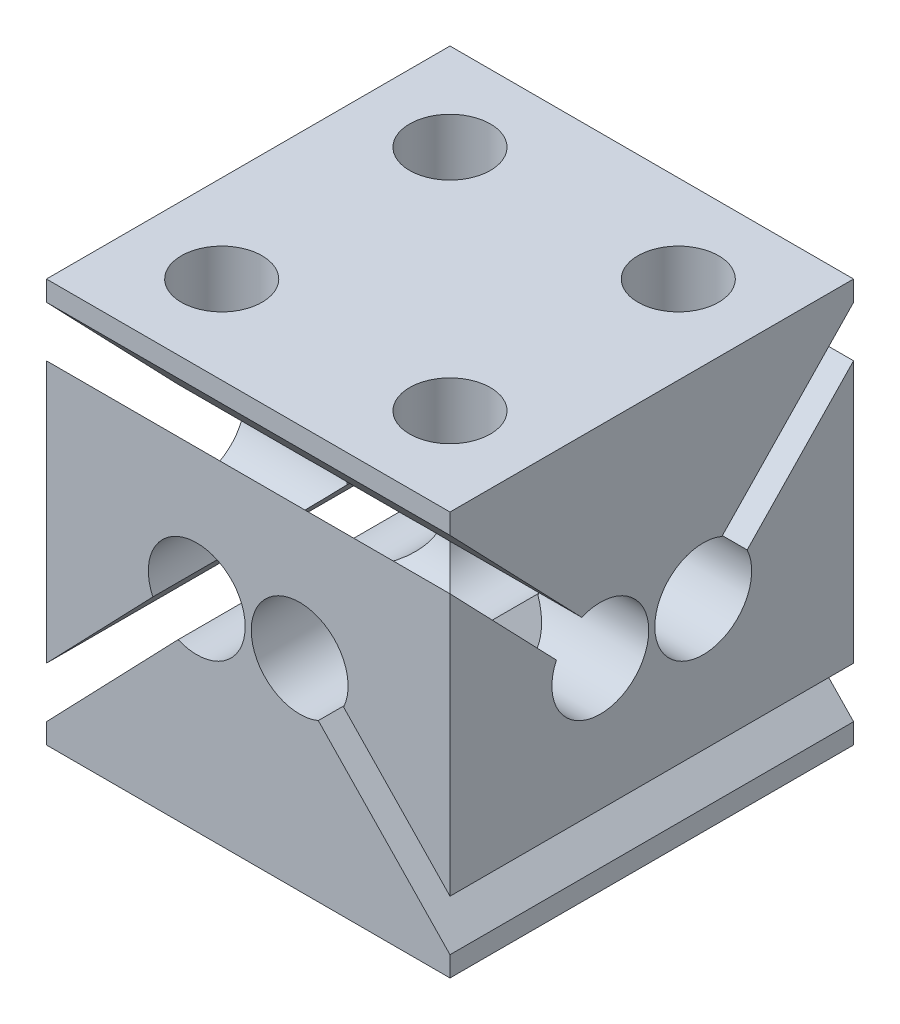
SolidWorks part; units mm, degrees
ref_plane "Front Plane" through (0, 0, 0) normal (0, 0, 1) x (1, 0, 0)
ref_plane "Top Plane" through (0, 0, 0) normal (0, 1, 0) x (1, 0, 0)
ref_plane "Right Plane" through (0, 0, 0) normal (1, 0, 0) x (0, 0, -1)
sketch "Sketch1" plane through (0, 0, 0) normal (0, 1, 0) x (1, 0, 0)
  line L1 (-5, -5) -> (5, -5)
  line L2 (-5, -5) -> (-5, 5)
  line L3 (-5, 5) -> (5, 5)
  line L4 (5, -5) -> (5, 5)
  line L5 (-5, -5) -> (5, 5) construction
  line L6 (-5, 5) -> (5, -5) construction
  point P0 (0, 0)
  dimension "D1" = 10
  dimension "D2" = 10
extrude "Boss-Extrude1" add sketch "Sketch1" along normal blind 10
sketch "Sketch2" plane through (0, 0, 5) normal (0, 0, 1) x (1, 0, 0)
  line L0 (-5, 0) -> (5, 0) construction
  line L1 (2.3638, 4.4955) -> (5, 1.755)
  line L2 (1.7368, 3.8924) -> (5, 0.5)
  line L4 (5, 1.755) -> (5, 0.5)
  line L5 (5, 10) -> (5, 0) construction
  line L6 (0, -1000) -> (0, 49000) construction
  line L7 (-5, 1.755) -> (-5, 0.5)
  line L8 (-1.7368, 3.8924) -> (-5, 0.5)
  line L9 (-2.3638, 4.4955) -> (-5, 1.755)
  arc A0 (-1.7368, 3.8924) -> (-2.3638, 4.4955) centre (-1.275, 5) ccw
  arc A1 (2.3638, 4.4955) -> (1.7368, 3.8924) centre (1.275, 5) ccw
  point P15 (0, 0)
  dimension "D1" = 2.4
  dimension "D3" = 0.87
  dimension "D4" = 5
  dimension "D5" = 1.275
  dimension "D7" = 0.5
  dimension "D6" = 0.435
extrude "Cut-Extrude1" cut sketch "Sketch2" against normal through all
sketch "Sketch3" plane through (5, 0, 0) normal (1, 0, 0) x (0, 0, -1)
  line L26 (-5, 8.245) -> (-5, 9.5)
  line L27 (5, 8.245) -> (5, 9.5)
  line L28 (1.7368, 6.1076) -> (5, 9.5)
  line L29 (2.3638, 5.5045) -> (5, 8.245)
  line L30 (5, 8.245) -> (5, 9.5)
  line L31 (1.7368, 6.1076) -> (5, 9.5)
  line L32 (2.3638, 5.5045) -> (5, 8.245)
  line L33 (5, 8.245) -> (5, 9.5)
  line L34 (1.7368, 6.1076) -> (5, 9.5)
  line L35 (2.3638, 5.5045) -> (5, 8.245)
  line L36 (5, 8.245) -> (5, 9.5)
  line L37 (1.7368, 6.1076) -> (5, 9.5)
  line L38 (2.3638, 5.5045) -> (5, 8.245)
  line L39 (-2.3638, 5.5045) -> (-5, 8.245)
  line L40 (-1.7368, 6.1076) -> (-5, 9.5)
  line L41 (-2.3638, 5.5045) -> (-5, 8.245)
  line L42 (-1.7368, 6.1076) -> (-5, 9.5)
  line L43 (-2.3638, 5.5045) -> (-5, 8.245)
  line L44 (-1.7368, 6.1076) -> (-5, 9.5)
  line L45 (-2.3638, 5.5045) -> (-5, 8.245)
  line L46 (-1.7368, 6.1076) -> (-5, 9.5)
  arc A8 (1.7368, 6.1076) -> (2.3638, 5.5045) centre (1.275, 5) ccw
  arc A9 (2.3638, 5.5045) -> (1.7368, 6.1076) centre (1.275, 5) cw
  arc A10 (1.7368, 6.1076) -> (2.3638, 5.5045) centre (1.275, 5) ccw
  arc A11 (2.3638, 5.5045) -> (1.7368, 6.1076) centre (1.275, 5) cw
  arc A12 (-2.3638, 5.5045) -> (-1.7368, 6.1076) centre (-1.275, 5) ccw
  arc A13 (-1.7368, 6.1076) -> (-2.3638, 5.5045) centre (-1.275, 5) cw
  arc A14 (-2.3638, 5.5045) -> (-1.7368, 6.1076) centre (-1.275, 5) ccw
  arc A15 (-1.7368, 6.1076) -> (-2.3638, 5.5045) centre (-1.275, 5) cw
  line M3 (-5, 10) -> (-5, 1.755)
  line M5 (5, 1.755) -> (5, 10)
  dimension "D1" = 0.5
  dimension "D2" = 0.5
extrude "Cut-Extrude2" cut sketch "Sketch3" against normal through all contours L28 A8 L29 M5 | L39 A12 L40 M3
sketch "Sketch4" plane through (0, 10, 0) normal (0, 1, 0) x (1, 0, 0)
  circle A0 centre (0, 0) radius 2.4592
sketch "Sketch5" plane through (0, 0, 0) normal (0, -1, 0) x (1, 0, 0)
  line L0 (0, 0) -> (-2.8459, 2.8108) construction
  line L1 (-2.8459, 2.8108) -> (2.8459, -2.8108) construction
  circle A0 centre (0, 0) radius 4 construction
  circle A1 centre (-2.8459, 2.8108) radius 0.6
  circle A2 centre (2.8459, -2.8108) radius 0.6
  dimension "D1" = 8
  dimension "D2" = 1.2
  dimension "D3" = 1.2
extrude "Cut-Extrude3" cut sketch "Sketch5" against normal blind 2
sketch "Sketch6" plane through (0, 10, 0) normal (0, 1, 0) x (1, 0, 0)
  line L0 (0, 0) -> (-2.8284, 2.8284) construction
  line L1 (0, 0) -> (0, 4) construction
  circle A0 centre (0, 0) radius 4 construction
  circle A1 centre (-2.8284, 2.8284) radius 1
  circle A2 centre (2.8284, 2.8284) radius 1
  circle A3 centre (2.8284, -2.8284) radius 1
  circle A4 centre (-2.8284, -2.8284) radius 1
  point P15 (0, 0)
  dimension "D1" = 8
  dimension "D3" = 2
  dimension "D2" = 45
  dimension "D4" = 4
extrude "Cut-Extrude4" cut sketch "Sketch6" against normal blind 1.5
